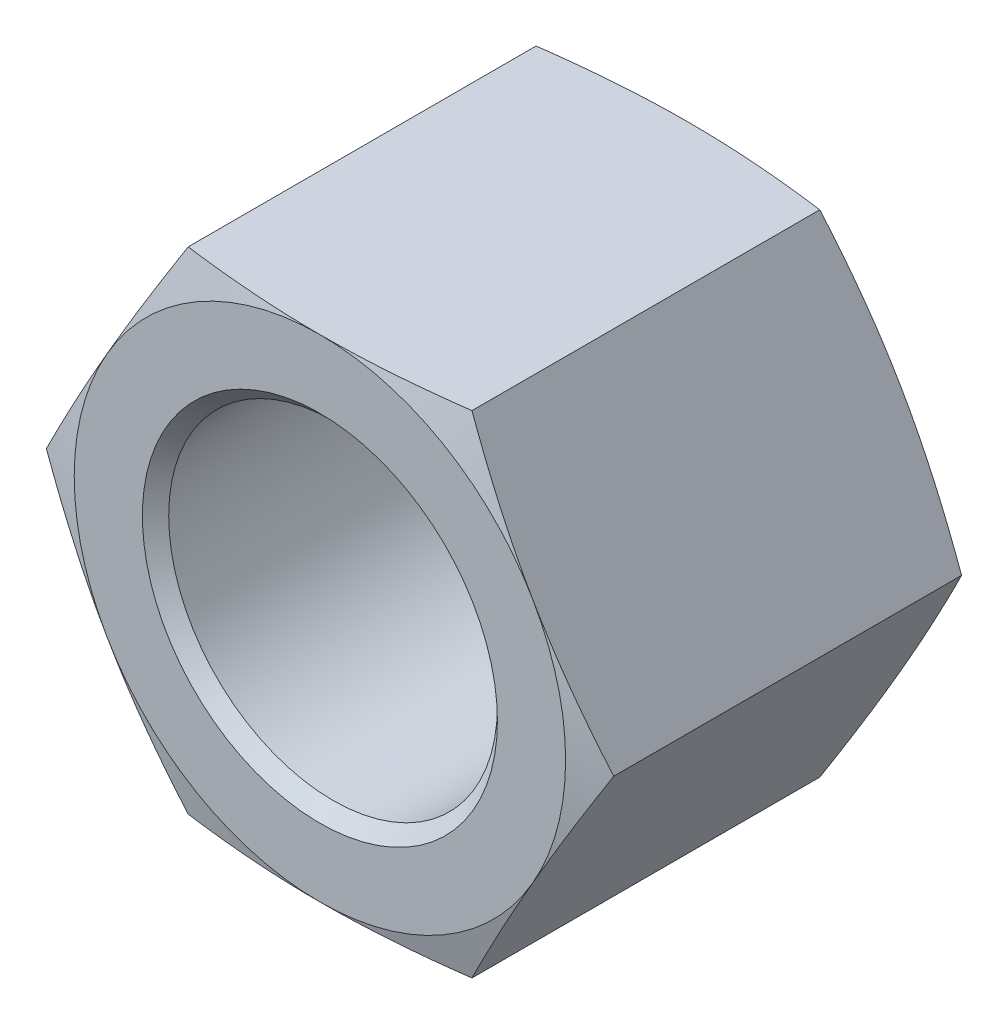
SolidWorks part; units mm, degrees
ref_plane "Plane1" through (0, 0, 0) normal (0, 0, 1) x (1, 0, 0)
ref_plane "Plane2" through (0, 0, 0) normal (0, 1, 0) x (1, 0, 0)
ref_plane "Plane3" through (0, 0, 0) normal (1, 0, 0) x (0, 0, -1)
sketch "Dimension Sketch" plane through (0, 0, 0) normal (0, 0, 1) x (1, 0, 0)
  line L0 (0, 0) -> (24.1005, 0)
  point P3 (5, 0)
  point P4 (1.5, 0)
  point P5 (8.63, 0)
  point P6 (5.6, 0)
  point P7 (6.4, 0)
  point P8 (8, 0)
sketch "Sketch1" plane through (0, 0, 0) normal (0, 0, 1) x (1, 0, 0)
  line L0 (-26.8088, 0) -> (37.1748, 0) construction
  line L1 (0, 25.0215) -> (0, -25.0215) construction
  line L3 (2.1575, 3.7369) -> (-2.1575, 3.7369)
  line L4 (-2.1575, 3.7369) -> (-4.315, 0)
  line L5 (-4.315, 0) -> (-2.1575, -3.7369)
  line L6 (-2.1575, -3.7369) -> (2.1575, -3.7369)
  line L7 (2.1575, -3.7369) -> (4.315, 0)
  line L8 (4.315, 0) -> (2.1575, 3.7369)
  circle A0 centre (0, 0) radius 3.7369 construction
  circle A1 centre (0, 0) radius 2.5
extrude "Boss-Extrude" add sketch "Sketch1" along normal blind 5.6
cosmetic thread "Cosmetic Thread1" parameters "D2"=5.25
sketch "Sketch2" plane through (0, 0, 0) normal (0, 0, -1) x (-1, 0, 0)
  line L0 (-2.1575, 3.7369) -> (2.1575, 3.7369) construction
  circle A0 centre (0, 0) radius 3.7369
  circle A1 centre (0, 0) radius 2.5 construction
extrude "Cut-Extrude1" cut sketch "Sketch2" against normal blind 38 draft 75 flip side to cut
sketch "Sketch3" plane through (0, 0, 5.6) normal (0, 0, 1) x (1, 0, 0)
  line L0 (4.315, 0) -> (2.1575, 3.7369) construction
  circle A0 centre (0, 0) radius 3.7369
extrude "Cut-Extrude2" cut sketch "Sketch3" against normal blind 38 draft 75 flip side to cut
chamfer "Chamfer1" distance 0.2 angle 45 2 edges at (2.5, 0, 0) (2.5, 0, 5.6)
equation "\"e@Sketch1\" = \"e@Dimension Sketch\""
equation "\"D@Sketch1\" = \"D@Dimension Sketch\""
equation "\"m@Boss-Extrude\" = \"m@Dimension Sketch\""
equation "\"D2@Cosmetic Thread1\" = 1.05 * \"D@Dimension Sketch\""
